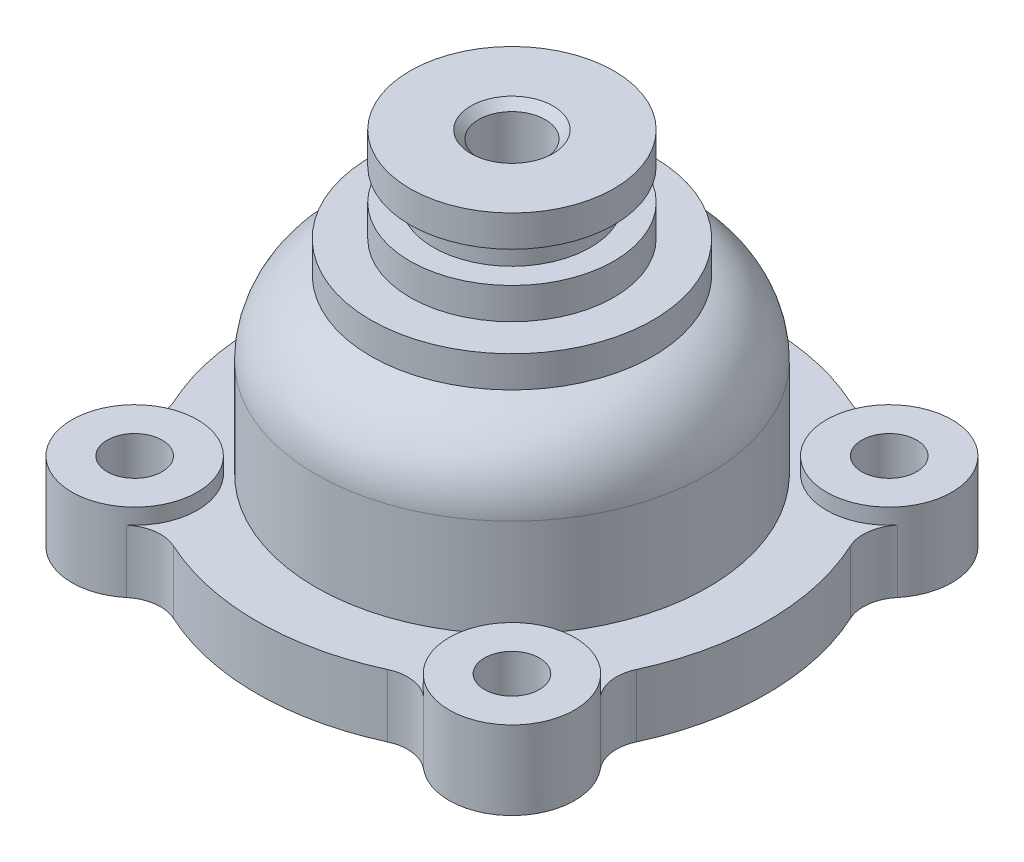
SolidWorks part; units mm, degrees
ref_plane "Front Plane" through (0, 0, 0) normal (0, 0, 1) x (1, 0, 0)
ref_plane "Top Plane" through (0, 0, 0) normal (0, 1, 0) x (1, 0, 0)
ref_plane "Right Plane" through (0, 0, 0) normal (1, 0, 0) x (0, 0, -1)
other "Configuration Table"
sketch "Sketch1" plane through (0, 0, 0) normal (0, 0, 1) x (1, 0, 0)
  line L0 (0, 0) -> (0, 27.1415) construction
  line L1 (0, 46) -> (-13, 46)
  line L2 (-13, 46) -> (-13, 42)
  line L3 (-13, 42) -> (-10, 42)
  line L4 (-10, 42) -> (-10, 38)
  line L5 (-10, 38) -> (-13, 38)
  line L6 (-13, 38) -> (-13, 34)
  line L7 (-13, 34) -> (-18, 34)
  line L8 (-18, 34) -> (-18, 30.0062)
  line L9 (-20, 0) -> (-20, 21)
  line L10 (-15, 26) -> (0, 26)
  line L11 (-20, 0) -> (-32.5, 0)
  line L12 (-32.5, 0) -> (-32.5, 8)
  line L13 (-32.5, 8) -> (-25, 8)
  line L14 (-25, 8) -> (-25, 20.4668)
  line L15 (0, 26) -> (0, 46)
  arc A0 (-18, 30.0062) -> (-25, 20.4668) centre (-15, 20.4668) ccw
  arc A1 (-20, 21) -> (-15, 26) centre (-15, 21) cw
  point P23 (-20, 26)
  dimension "D8" = 20
  dimension "D15" = 5
  dimension "D1" = 13
  dimension "D2" = 3
  dimension "D3" = 3
  dimension "D4" = 4
  dimension "D5" = 4
  dimension "D6" = 4
  dimension "D7" = 18
  dimension "D9" = 46
  dimension "D10" = 26
  dimension "D11" = 20
  dimension "D12" = 8
  dimension "D13" = 32.5
  dimension "D14" = 5
revolve "Revolve1" add sketch "Sketch1" angle 360 about L0
sketch "Sketch4" plane through (0, 46, 0) normal (0, 1, 0) x (1, 0, 0)
  point P0 (0, 0)
hole_wizard "M10 Tapped Hole1" positions "Sketch4" profile "Sketch5" tap size "M10" standard "GB" end condition through all
sketch "Sketch5" plane through (0, 46, 0) normal (1, 0, 0) x (0, 0, 1)
  line L0 (0, 0) -> (0, 46)
  line L1 (0, 46) -> (4.25, 46)
  line L2 (4.25, 46) -> (4.25, 0)
  line L5 (4.25, 0) -> (0, 0)
  line L11 (0, -6.35) -> (0, 107.95) construction
  dimension "通孔螺纹孔钻头直径" = 8.5
  dimension "通孔螺纹孔钻头深度" = 46
cosmetic thread "Cosmetic Thread1" parameters "D2"=10
chamfer "Chamfer1" distance 1 angle 45 1 edges at (0, 46, 4.25)
sketch "Sketch6" plane through (0, 8, 0) normal (0, 1, 0) x (1, 0, 0)
  line L0 (0, 0) -> (0, 34.7565) construction
  line L1 (0, 0) -> (-28.0982, 28.0982) construction
  circle A0 centre (0, 0) radius 34 construction
  circle A1 centre (-24.0416, 24.0416) radius 8
  circle A2 centre (24.0416, 24.0416) radius 8
  circle A3 centre (24.0416, -24.0416) radius 8
  circle A4 centre (-24.0416, -24.0416) radius 8
  circle A5 centre (-24.0416, 24.0416) radius 3.5
  circle A6 centre (24.0416, 24.0416) radius 3.5
  circle A7 centre (24.0416, -24.0416) radius 3.5
  circle A8 centre (-24.0416, -24.0416) radius 3.5
  point P16 (0, 0)
  point P24 (0, 0)
  dimension "D2" = 68
  dimension "D3" = 16
  dimension "D5" = 7
  dimension "D1" = 45
  dimension "D4" = 4
  dimension "D6" = 4
extrude "Boss-Extrude1" add sketch "Sketch6" against normal blind 8
sketch "Sketch7" plane through (0, 8, 0) normal (0, 1, 0) x (1, 0, 0)
  line L0 (0, 0) -> (0, 35.2246) construction
  circle A0 centre (-24.0416, 24.0416) radius 3.5
  arc A1 (-20.6933, 25.0607) -> (-25.0607, 20.6933) centre (-24.0416, 24.0416) ccw construction
  circle A2 centre (24.0416, 24.0416) radius 3.5
  circle A3 centre (24.0416, -24.0416) radius 3.5
  circle A4 centre (-24.0416, -24.0416) radius 3.5
  point P17 (0, 0)
  dimension "D1" = 4
extrude "Cut-Extrude1" cut sketch "Sketch7" against normal blind 8
fillet "Fillet1" radius 5 8 edges at (-16.9444, 4, -27.7333) (-27.7333, 4, -16.9444) (27.7333, 4, -16.9444) (16.9444, 4, -27.7333) (16.9444, 4, 27.7333) (27.7333, 4, 16.9444) (-27.7333, 4, 16.9444) (-16.9444, 4, 27.7333)
sketch "Sketch8" plane through (0, 8, 0) normal (0, 1, 0) x (1, 0, 0)
  circle A0 centre (-24.0416, 24.0416) radius 8
  circle A1 centre (24.0416, 24.0416) radius 8
  circle A2 centre (24.0416, -24.0416) radius 8
  circle A3 centre (-24.0416, -24.0416) radius 8
  circle A4 centre (-24.0416, -24.0416) radius 3.5 construction
  circle A5 centre (24.0416, -24.0416) radius 3.5 construction
  circle A6 centre (-24.0416, 24.0416) radius 3.5 construction
  circle A7 centre (24.0416, 24.0416) radius 3.5 construction
  circle A8 centre (-24.0416, -24.0416) radius 3.5
  circle A9 centre (24.0416, -24.0416) radius 3.5
  circle A10 centre (-24.0416, 24.0416) radius 3.5
  circle A11 centre (24.0416, 24.0416) radius 3.5
  point P12 (0, 0)
  dimension "D1" = 16
  dimension "D2" = 4
extrude "Boss-Extrude2" add sketch "Sketch8" along normal blind 2
